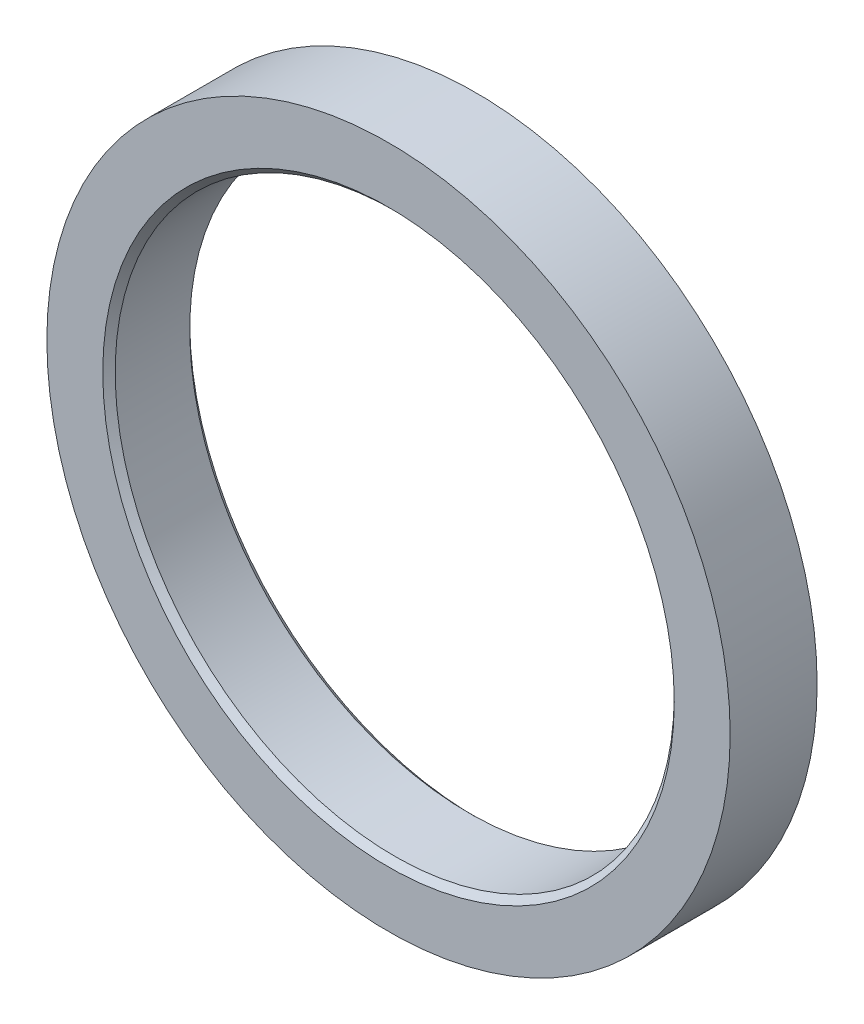
SolidWorks part; units mm, degrees
ref_plane "Front Plane" through (0, 0, 0) normal (0, 0, 1) x (1, 0, 0)
ref_plane "Top Plane" through (0, 0, 0) normal (0, 1, 0) x (1, 0, 0)
ref_plane "Right Plane" through (0, 0, 0) normal (1, 0, 0) x (0, 0, -1)
ref_plane "Plane1" through (0, 22.744, 0) normal (0, 1, 0) x (1, 0, 0)
sketch "Sketch1" plane through (0, 22.744, 0) normal (0, 1, 0) x (1, 0, 0)
  line L0 (598.7306, 329.193) -> (599.2306, 328.693)
  line L1 (599.2306, 328.693) -> (603.7306, 328.693)
  line L2 (603.7306, 328.693) -> (603.7306, 335.693)
  line L3 (603.7306, 335.693) -> (599.2306, 335.693)
  line L4 (599.2306, 335.693) -> (598.7306, 335.193)
  line L5 (598.7306, 335.193) -> (598.7306, 329.193)
  line L6 (576.2306, 335.693) -> (576.2306, 328.693) construction
  dimension "D1" = 22.5
  dimension "D2" = 23
  dimension "D3" = 27.5
  dimension "D4" = 0.5
  dimension "D5" = 6.5
  dimension "D6" = 7
revolve "Revolve1" add sketch "Sketch1" angle 360 about L6
